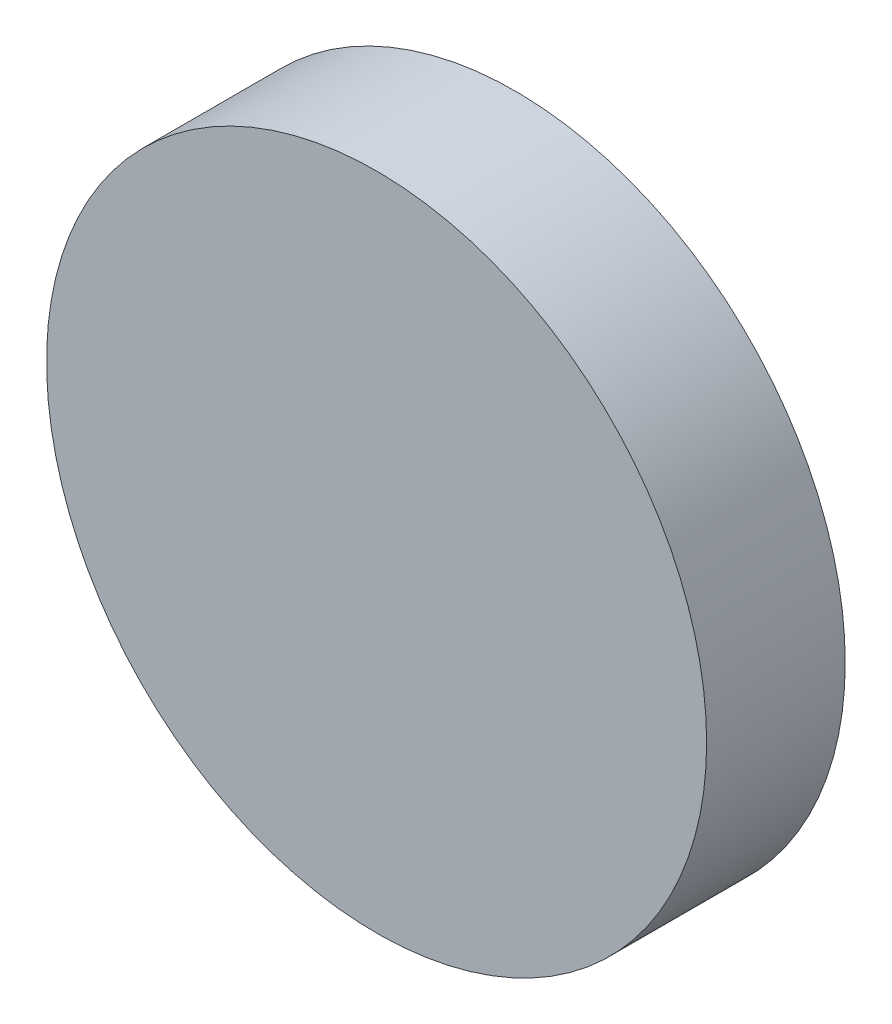
from build123d import *

# Parameters (mm, degrees)
SKETCH1_R           = 250
BOSS_EXTRUDE1_DEPTH = 105


with BuildPart() as part:
    # Sketch1 → Boss-Extrude1 (new body)
    with BuildSketch(Plane.XY):
        Circle(SKETCH1_R)
    extrude(amount=BOSS_EXTRUDE1_DEPTH)


solid = part.part
